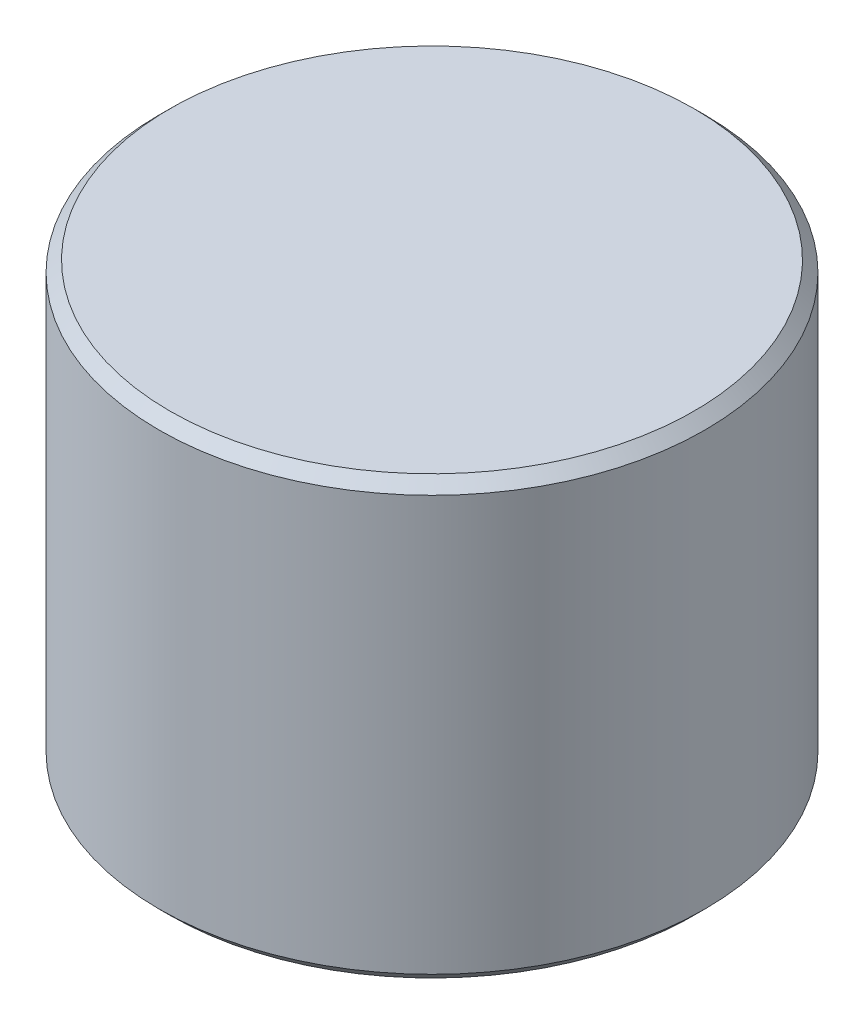
from build123d import *

# Parameters (mm, degrees)
SKETCH1_R           = 5
BOSS_EXTRUDE1_DEPTH = 8
CHAMFER1_SIZE       = 0.2


with BuildPart() as part:
    # Sketch1 → Boss-Extrude1 (new body)
    with BuildSketch(Plane(origin=(0, 0, 0), x_dir=(1, 0, 0), z_dir=(0, 1, 0))):
        with Locations(Location((0, 0, 0), (0, 0, 270))):
            Circle(SKETCH1_R)
    extrude(amount=BOSS_EXTRUDE1_DEPTH)

    # Chamfer1
    chamfer1_edges = [part.edges().sort_by_distance(p)[0] for p in [
        (0, 0, -5),
        (0, 8, -5),
    ]]
    chamfer(chamfer1_edges, length=CHAMFER1_SIZE)


solid = part.part
